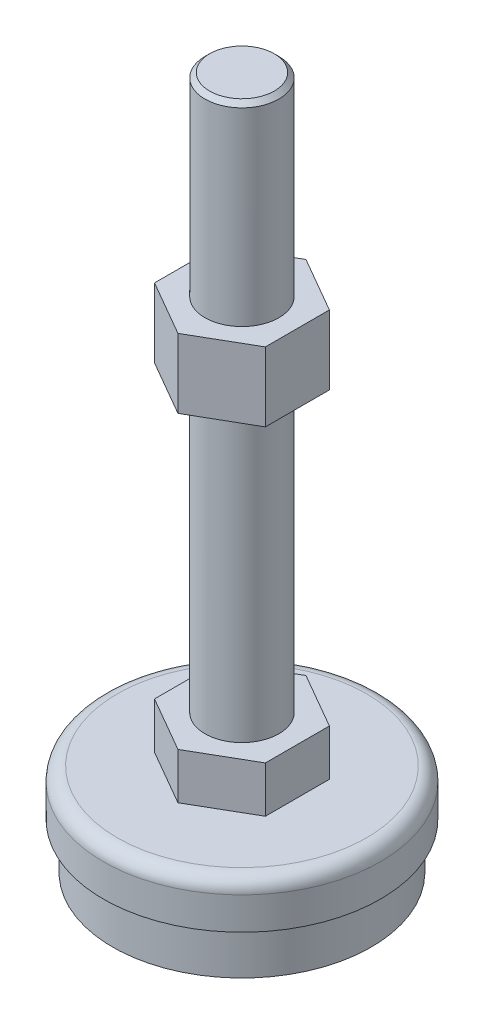
SolidWorks part; units mm, degrees
ref_plane "前视" through (0, 0, 0) normal (0, 0, 1) x (1, 0, 0)
ref_plane "上视" through (0, 0, 0) normal (0, 1, 0) x (1, 0, 0)
ref_plane "右视" through (0, 0, 0) normal (1, 0, 0) x (0, 0, -1)
sketch "草图1" plane through (0, 0, 0) normal (0, 0, 1) x (1, 0, 0)
  line L0 (0, 0) -> (0, 232.4997) construction
  line L1 (0, 0) -> (0, 150)
  line L2 (0, 150) -> (8, 150)
  line L3 (8, 150) -> (8, 20)
  line L4 (8, 20) -> (27, 20)
  line L5 (30, 17) -> (30, 10)
  line L6 (28, 0) -> (0, 0)
  line L7 (30, 10) -> (28, 10)
  line L8 (28, 10) -> (28, 0)
  line L9 (8, 30) -> (27, 30) construction
  arc A0 (27, 20) -> (30, 17) centre (27, 17) cw
  point P12 (30, 20)
  dimension "D7" = 3
  dimension "D1" = 60
  dimension "D2" = 20
  dimension "D3" = 16
  dimension "D4" = 10
  dimension "D5" = 2
  dimension "D6" = 10
  dimension "D8" = 120
revolve "旋转1" add sketch "草图1" angle 360 about L0
sketch "草图2" plane through (0, 20, 0) normal (0, 1, 0) x (1, 0, 0)
  line L1 (0, 13.8564) -> (-12, 6.9282)
  line L2 (-12, 6.9282) -> (-12, -6.9282)
  line L3 (-12, -6.9282) -> (0, -13.8564)
  line L4 (0, -13.8564) -> (12, -6.9282)
  line L5 (12, -6.9282) -> (12, 6.9282)
  line L6 (12, 6.9282) -> (0, 13.8564)
  circle A0 centre (0, 0) radius 12 construction
  circle A1 centre (0, 0) radius 8 construction
  circle A2 centre (0, 0) radius 8
  dimension "D1" = 24
extrude "凸台-拉伸1" add sketch "草图2" along normal blind 10 separate body
sketch "草图4" plane through (0, 30, 0) normal (0, 1, 0) x (1, 0, 0)
  line L6 (12, 6.9282) -> (0, 13.8564)
  line L7 (0, 13.8564) -> (-12, 6.9282)
  line L8 (-12, 6.9282) -> (-12, -6.9282)
  line L9 (-12, -6.9282) -> (0, -13.8564)
  line L10 (0, -13.8564) -> (12, -6.9282)
  line L11 (12, -6.9282) -> (12, 6.9282)
  line L12 (12, 6.9282) -> (0, 13.8564)
  line L13 (0, 13.8564) -> (-12, 6.9282)
  line L14 (-12, 6.9282) -> (-12, -6.9282)
  line L15 (-12, -6.9282) -> (0, -13.8564)
  line L16 (0, -13.8564) -> (12, -6.9282)
  line L17 (12, -6.9282) -> (12, 6.9282)
  dimension "D1" = 0
extrude "凸台-拉伸2" add sketch "草图4" along normal blind 15 from offset 63 separate body
chamfer "倒角1" distance 1 angle 45 1 edges at (0, 150, -8)
